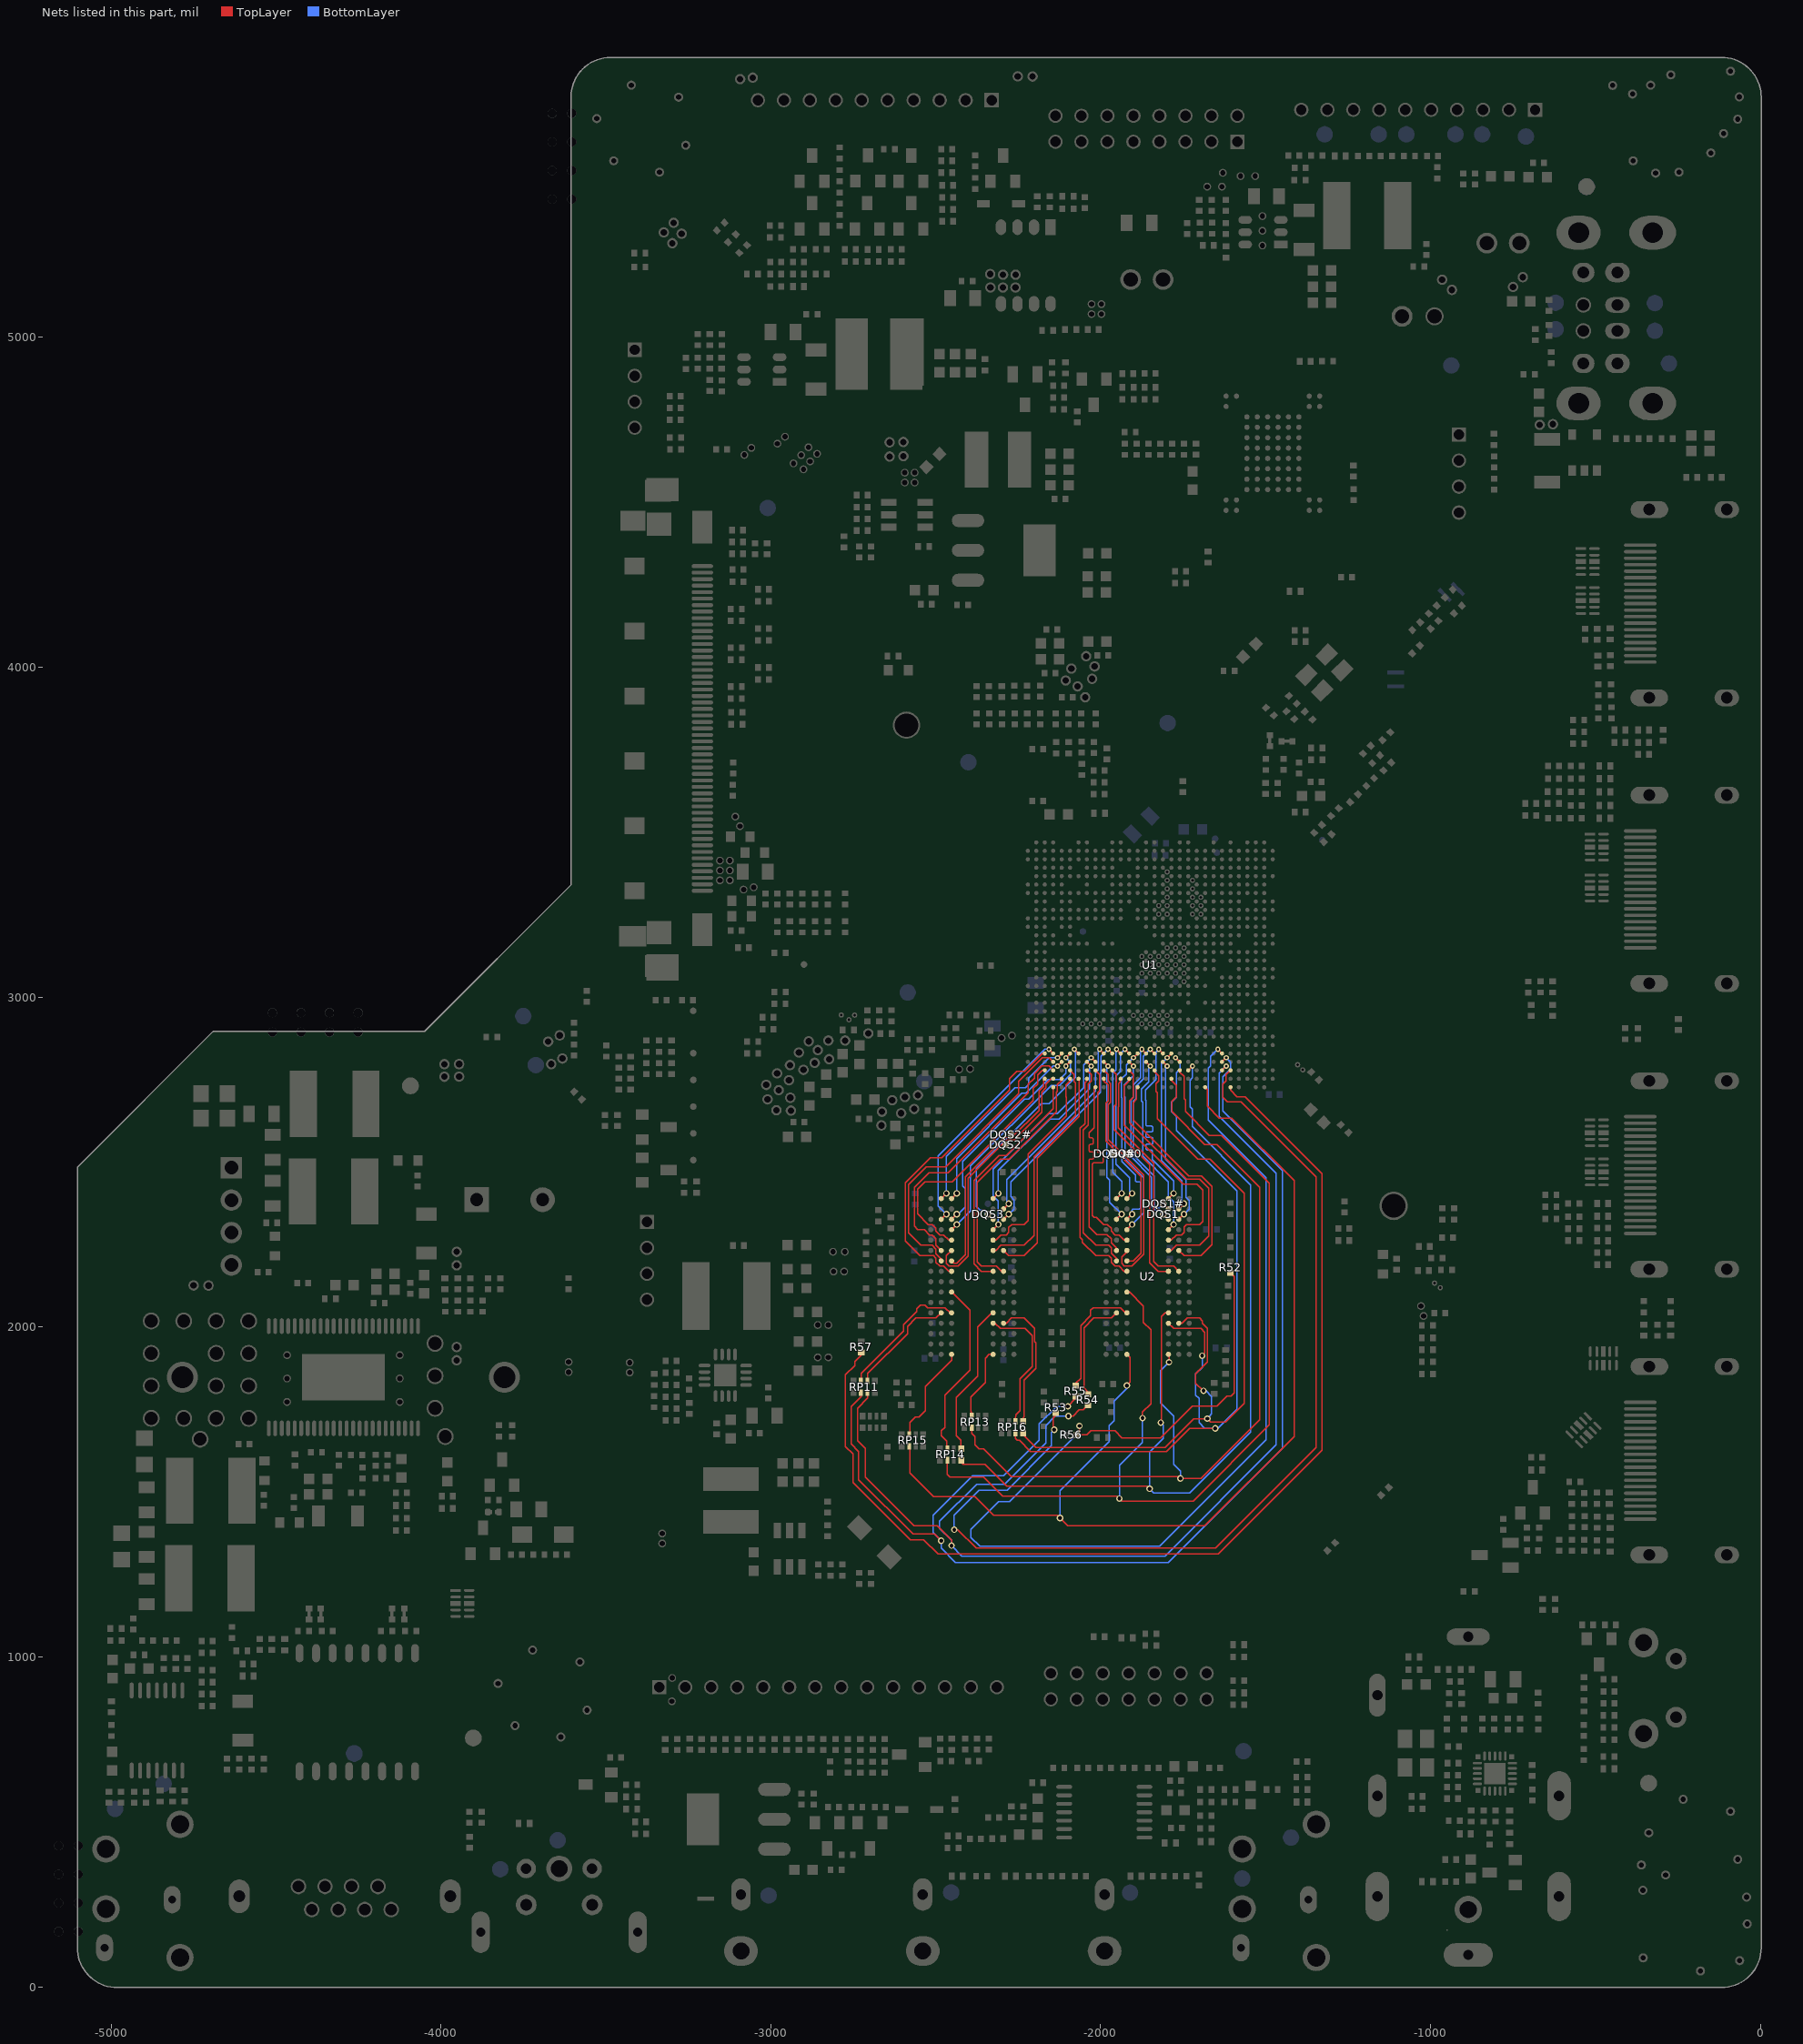
[diagram p0: the nets of this part, all layers, seen from the top]
# Altium PCB MISC86290.PcbDoc (part 12 of 31)
Units mil, origin at the board's own origin, x right, y up, seen from the top; angles counter-clockwise.
Board outline 5104.71 x 5851.49 mil, 2 copper layers (TopLayer, BottomLayer), stack 61.855 mil thick; 1026 components, 667 nets, 4280 pads, 2294 vias.

## Via types
v1: diameter 19.68, hole 11.81, TopLayer to BottomLayer, tented both sides, 1189 vias
v2: diameter 19.68/19.68 (per signal layer), hole 11.81, TopLayer to BottomLayer, tented both sides, 366 vias
v3: diameter 15.75, hole 7.87, TopLayer to BottomLayer, tented both sides, 348 vias
v4: diameter 23.62, hole 15.75, TopLayer to BottomLayer, tented both sides, 309 vias
v5: diameter 15.75/15.75 (per signal layer), hole 7.87, TopLayer to BottomLayer, tented both sides, 59 vias
v6: diameter 24/24 (per signal layer), hole 16, TopLayer to BottomLayer, tented both sides, 23 vias

## Nets (pads, with @x,y where several pads share a name; then routed paths per layer and width w, separated by ;. In a path a pad name is that pad's centre, name@x,y a point inside that pad or via, vN(x,y) a via of type N, cw(c..) or ccw(c..) an arc to the next point about the centre after c; other vN are vias at no path point) (continued)
D_DDR3_A12: RP16.4 U1.D12 U2.N7 | length 2408.7
  TopLayer w3.94: RP16.4@-2259.17,1678.74 -2259.17,1662.01 -2253.27,1656.1 -2246.38,1656.1 -2212.91,1622.64 -1800.51,1622.64 -1730.63,1692.52 v2(-1652.87,1692.52) ; U2.N7@-1794.61,2011.42 -1778.86,1995.67 -1696.18,1995.67 -1684.37,1983.86 -1684.37,1920.87 v2(-1692.24,1912.99) ; v5(-1772.95,2816.54) U1.D12@-1760.16,2803.74
  BottomLayer w3.94: v5(-1772.95,2816.54) -1759.17,2802.76 -1759.17,2783.07 -1770.98,2771.26 -1770.98,2696.46 -1785.75,2681.69 -1785.75,2653.15 -1770.98,2638.39 -1770.98,2596.06 -1586.93,2412.01 -1586.93,1750.59 -1645,1692.52 v2(-1652.87,1692.52) -1684.37,1692.52 -1702.09,1710.24 -1702.09,1783.07 -1711.93,1792.91 -1711.93,1857.87 -1692.24,1877.56 v2(-1692.24,1912.99)
D_DDR3_A12_H: RP16.3 U3.N7 | length 406.1
  TopLayer w3.94: U3.N7@-2326.1,2011.42 -2320.2,2011.42 -2304.45,1995.67 -2229.65,1995.67 -2207.99,1974.02 -2207.99,1879.53 -2244.41,1843.11 -2244.41,1746.65 -2257.2,1733.86 RP16.3@-2259.17,1722.05
D_DDR3_A13: RP15.6 U1.A9 U2.T3 | length 3206
  TopLayer w3.94: RP15.6@-2579.06,1638.39 -2579.06,1557.68 -2507.2,1485.83 -2381.22,1485.83 -2324.13,1428.74 -2131.22,1428.74 v2(-2123.35,1420.87) -2099.72,1397.24 -1684.37,1397.24 -1413.7,1667.91 -1413.7,2443.5 -1603.66,2633.46 -1641.06,2633.46 -1677.27,2669.68 -1677.27,2686.35 -1676.5,2687.13 -1676.5,2720.08 U1.A9@-1683.39,2726.97 ; v2(-1920.59,1822.44) -1920,1823.82 -1910.75,1833.07 -1910.75,1907.09 U2.T3@-1920.59,1916.93
  BottomLayer w3.94: v2(-2123.35,1420.87) -2123.35,1503.54 -1974.72,1652.17 -1974.72,1701.38 -1959.96,1716.14 -1959.96,1775.2 -1920.59,1814.57 v2(-1920.59,1822.44)
D_DDR3_A13_H: RP15.5 U3.T3 | length 294.2
  TopLayer w3.94: RP15.5@-2579.06,1681.69 -2579.06,1710.24 -2562.32,1726.97 -2551.5,1726.97 -2531.81,1746.65 -2531.81,1819.49 -2452.09,1899.21 U3.T3@-2452.09,1916.93
D_DDR3_A14: RP13.6 U1.B13 U2.T7 | length 2625.8
  TopLayer w3.94: RP13.6@-2391.06,1694.49 -2391.06,1677.76 -2381.22,1667.91 -2381.22,1643.31 -2368.43,1630.51 -2355.63,1630.51 -2270.98,1545.87 -1763.11,1545.87 v2(-1758.19,1540.94) -1696.18,1540.94 -1518.03,1719.09 -1518.03,2423.82 -1646.97,2552.76 -1684.37,2552.76 -1784.76,2653.15 -1784.76,2684.65 -1770.98,2698.43 -1770.98,2732.91 U1.B13@-1785.71,2747.64 ; U2.T7@-1794.61,1916.93 -1792.64,1916.93 v2(-1792.64,1893.31) ; U1.B13@-1785.75,2747.64 U1.B13@-1785.75,2752.56
  BottomLayer w3.94: v2(-1792.64,1893.31) -1818.23,1867.72 -1818.23,1769.29 -1778.86,1729.92 -1778.86,1583.27 -1758.19,1562.6 v2(-1758.19,1540.94)
D_DDR3_A14_H: RP13.5 U3.T7 | length 215.4
  TopLayer w3.94: RP13.5@-2391.06,1737.8 -2391.06,1740.07 -2394.02,1743.02 -2394.02,1787.99 -2349.72,1832.28 -2349.72,1905.12 -2337.91,1916.93 U3.T7@-2326.1,1916.93
D_DDR3_A15: RP14.2 U1.C11 U2.M7 | length 2781
  TopLayer w3.94: RP14.2@-2423.54,1596.06 -2423.54,1590.16 -2416.65,1583.27 -2350.71,1583.27 -2284.76,1517.32 -1859.57,1517.32 v2(-1851.69,1509.45) ; v2(-1818.23,1710.24) -1816.26,1707.36 -1816.26,2031.1 -1804.45,2042.91 U2.M7@-1794.61,2042.91 ; U1.C11@-1734.57,2778.15 v5(-1721.77,2790.94)
  BottomLayer w3.94: v2(-1818.23,1710.24) -1810.35,1702.36 -1810.35,1662.01 -1851.69,1620.67 v2(-1851.69,1509.45) -1838.9,1496.65 -1730.63,1496.65 -1545.59,1681.69 -1545.59,2430.71 -1722.76,2607.87 -1722.76,2660.04 -1729.65,2666.93 -1729.65,2747.64 -1721.77,2755.51 v5(-1721.77,2790.94)
D_DDR3_A15_H: RP14.1 U3.M7 | length 458.4
  TopLayer w3.94: RP14.1@-2423.54,1639.37 -2423.54,1656.1 -2438.31,1670.87 -2438.31,1786.02 -2373.35,1850.98 -2373.35,1999.61 -2330.04,2042.91 U3.M7@-2326.1,2042.91
D_DDR3_BA0: R54.2 RP11.4 U1.C7 | length 3734.8
  TopLayer w3.94: RP11.4@-2706.02,1800.79 -2706.02,1785.04 -2737.5,1753.56 -2737.5,1655.1 -2713.9,1631.5 -2713.9,1544.88 -2566.26,1397.24 -2495.39,1397.24 -2452.09,1353.94 v2(-2452.09,1337.2) ; v2(-2097.76,1729.92) -2083.98,1729.92 -2065.3,1748.6 -2053.18,1748.6 R54.2@-2038.7,1763.07 ; U1.C7@-1632.2,2778.15 v3(-1619.41,2790.94)
  BottomLayer w3.94: v2(-2097.76,1729.92) -2138.11,1729.92 -2166.65,1701.38 -2166.65,1648.23 -2291.65,1523.23 -2376.3,1523.23 -2488.5,1411.02 -2488.5,1389.37 -2452.09,1352.95 v2(-2452.09,1337.2) -2420.59,1305.71 -1805.43,1305.71 -1468.82,1642.32 -1468.82,2466.14 -1641.06,2638.39 -1641.06,2769.29 v3(-1619.41,2790.94)
D_DDR3_BA0_H: RP11.3 U3.M2 | length 326.7
  TopLayer w3.94: RP11.3@-2706.02,1844.09 -2706.02,1859.84 -2585.94,1979.92 -2585.94,2001.57 -2560.35,2027.17 -2499.33,2027.17 U3.M2@-2483.58,2042.91
D_DDR3_BA0_L: R54.1 U2.M2 | length 316.6
  TopLayer w3.94: R54.1@-2038.7,1803.07 -2050.51,1814.88 -2050.51,1997.64 -2020.98,2027.17 -1967.83,2027.17 U2.M2@-1952.09,2042.91
D_DDR3_BA1: RP16.2 U1.C15 U2.N8 | length 2335
  TopLayer w3.94: RP16.2@-2236.54,1678.74 -2236.52,1678.64 -2236.07,1674.34 -2196.18,1634.45 -1805.43,1634.45 -1717.83,1722.05 v2(-1676.5,1722.05) -1666.65,1712.2 -1621.38,1712.2 -1565.28,1768.31 -1565.28,2406.1 -1668.62,2509.45 -1706.02,2509.45 -1828.07,2631.5 -1828.07,2710.24 -1832.5,2714.67 -1832.5,2737.3 -1824.13,2745.67 -1824.13,2761.42 -1836.93,2774.21 U1.C15@-1836.93,2778.15 ; U2.N8@-1763.11,2011.42 -1753.27,2011.42 -1737.52,2027.17 -1700.12,2027.17 -1691.26,2018.31 -1691.26,2010.43 -1676.5,1995.67 -1676.5,1893.31 -1711.93,1857.87 -1711.93,1829.33 -1689.29,1806.69 v2(-1688.31,1806.69)
  BottomLayer w3.94: v2(-1688.31,1806.69) -1681.42,1806.69 -1663.7,1788.98 -1663.7,1736.81 v2(-1676.5,1722.05)
D_DDR3_BA1_H: RP16.1 U3.N8 | length 405.8
  TopLayer w3.94: U3.N8@-2294.61,2011.42 -2286.73,2011.42 -2270.98,2027.17 -2231.61,2027.17 -2200.12,1995.67 -2200.12,1956.3 -2196.18,1952.36 -2196.18,1874.61 -2232.6,1838.19 -2232.6,1726.97 -2234.57,1725 RP16.1@-2236.54,1722.05
D_DDR3_BA2: R55.2 RP11.6 U1.D7 | length 3823.5
  TopLayer w3.94: RP11.6@-2725.71,1800.79 -2725.71,1788.98 -2756.22,1758.46 -2756.22,1645.28 -2733.58,1622.64 -2733.58,1537.01 -2569.21,1372.64 -2504.25,1372.64 v2(-2483.58,1351.97) ; v2(-2099.72,1759.45) -2076.1,1783.07 R55.2@-2076.1,1788.66 ; U1.D7@-1632.2,2803.74 v5(-1619.41,2816.54)
  BottomLayer w3.94: v2(-2099.72,1759.45) -2133.19,1759.45 -2186.34,1706.3 -2186.34,1657.09 -2294.11,1549.31 -2387.62,1549.31 -2508.19,1428.74 -2508.19,1376.57 v2(-2483.58,1351.97) -2483.58,1329.33 -2440.28,1286.02 -1795.59,1286.02 -1449.13,1632.48 -1449.13,2475 -1629.25,2655.12 -1629.25,2758.46 -1605.63,2782.09 -1605.63,2802.76 v5(-1619.41,2816.54)
D_DDR3_BA2_H: RP11.5 U3.M3 | length 397
  TopLayer w3.94: RP11.5@-2725.72,1844.11 -2725.72,1859.83 -2597.76,1987.8 -2597.76,2007.48 -2558.39,2046.85 -2558.39,2054.72 -2546.57,2066.54 -2532.8,2066.54 -2524.92,2058.66 -2471.77,2058.66 U3.M3@-2456.02,2042.91
D_DDR3_BA2_L: R55.1 U2.M3 | length 360.9
  TopLayer w3.94: R55.1@-2076.1,1828.66 -2060.35,1844.41 -2060.35,2004.53 -2030.83,2034.06 -2030.83,2050.79 -2022.95,2058.66 -1940.28,2058.66 -1924.53,2042.91 U2.M3@-1920.59,2042.91
D_DDR3_CASZ: RP14.6 U1.C12 U2.K3 | length 3058.9
  TopLayer w3.94: RP14.6@-2465.87,1596.06 -2465.87,1553.74 -2457.01,1544.88 -2354.65,1544.88 -2297.56,1487.8 -1951.1,1487.8 v2(-1943.23,1479.92) -1935.35,1472.05 -1719.8,1472.05 -1488.5,1703.35 -1488.5,2435.63 -1633.19,2580.31 -1670.59,2580.31 -1743.43,2653.15 -1743.43,2688.58 -1747.36,2692.52 -1747.36,2759.45 -1760.16,2772.24 U1.C12@-1760.16,2778.15 ; U2.K3@-1920.59,2105.91 -1912.72,2105.91 -1870.39,2063.58 -1870.39,2014.37 -1847.76,1991.73 -1847.76,1767.32 -1873.35,1741.73 v2(-1873.35,1724.02)
  BottomLayer w3.94: v2(-1943.23,1479.92) -1943.23,1580.31 -1874.33,1649.21 -1874.33,1723.03 v2(-1873.35,1724.02)
D_DDR3_CASZ_H: RP14.5 U3.K3 | length 532.3
  TopLayer w3.94: RP14.5@-2465.87,1639.37 -2466.86,1639.37 -2466.86,1654.14 -2482.6,1669.88 -2482.6,1685.63 -2472.76,1695.47 -2472.76,1793.9 -2396.97,1869.69 -2396.97,2050.79 U3.K3@-2452.09,2105.91
D_DDR3_CKE: R52.2 R56.1 U1.E7 | length 3759
  TopLayer w3.94: v2(-2064.29,1700.39) -2064.29,1674.49 -2065.94,1672.83 -2042.64,1672.83 -2029.84,1685.63 -1957.01,1685.63 -1935.35,1663.98 -1818.23,1663.98 -1721.77,1760.43 -1647.95,1760.43 -1617.44,1790.94 -1604.65,1790.94 -1594.8,1800.79 -1594.8,2153.15 -1605.63,2163.98 -1605.94,2163.98 R52.2@-1606.61,2164.65 ; v5(-1645,2842.13) U1.E7@-1632.2,2829.33
  BottomLayer w3.94: v2(-2064.29,1700.39) -2064.29,1682.68 -2276.89,1470.08 -2309.37,1470.08 -2393.03,1386.42 -2393.03,1361.81 -2366.46,1335.24 -1821.18,1335.24 -1498.35,1658.07 -1498.35,2452.36 -1673.54,2627.56 -1673.54,2785.04 -1666.65,2791.93 -1666.65,2820.47 v5(-1645,2842.13)
D_DDR3_CSB1: R53.2 U1.C6 | length 3069.4
  TopLayer w3.94: v2(-2444.21,1385.43) -2433.39,1385.43 -2377.28,1329.33 -1651.89,1329.33 -1346.77,1634.45 -1346.77,2455.31 -1574.13,2682.68 -1615.47,2682.68 -1629.25,2696.46 -1629.25,2735.83 -1619.41,2745.67 -1619.41,2765.35 U1.C6@-1606.61,2778.15 ; v2(-2141.06,1688.58) -2144.69,1688.58 -2144.69,1724.02 R53.2@-2137.13,1731.57
  BottomLayer w3.94: v2(-2444.21,1385.43) -2444.21,1429.72 -2368.43,1505.51 -2283.78,1505.51 -2148.94,1640.35 -2148.94,1680.71 v2(-2141.06,1688.58)
D_DDR3_CSB2: R57.1 U1.A6 | length 3289.4
  TopLayer w3.94: R57.1@-2724.72,1916.2 -2745.39,1895.53 -2745.39,1883.46 -2773.94,1854.92 -2773.94,1637.4 -2751.3,1614.76 -2751.3,1529.13 -2577.09,1354.92 -2536.73,1354.92 -2493.43,1311.61 -1644.02,1311.61 -1329.06,1626.57 -1329.06,2465.16 -1562.32,2698.43 -1586.93,2698.43 -1606.61,2718.11 U1.A6@-1606.61,2726.97
D_DDR3_DM0: U1.B18 U2.E7 | length 700.1
  TopLayer w3.94: U1.B18@-1913.7,2752.56 -1913.7,2746.65 -1929.45,2730.91 -1929.45,2611.81 -1750.32,2432.68 -1707.99,2432.68 -1690.28,2414.96 -1690.28,2320.47 -1700.12,2310.63 -1740.28,2310.63 -1747.36,2303.55 -1747.36,2287.01 -1755.24,2279.13 -1770.98,2279.13 -1786.73,2263.39 U2.E7@-1794.61,2263.39
D_DDR3_DM1: U1.D18 U2.D3 | length 571.2
  TopLayer w3.94: U2.D3@-1920.59,2294.88 v2(-1904.84,2310.63) ; U1.D18@-1913.7,2803.74 v5(-1900.91,2790.94)
  BottomLayer w3.94: v2(-1904.84,2310.63) -1869.41,2346.06 -1869.41,2452.36 -1926.5,2509.45 -1926.5,2697.44 -1928.46,2699.41 -1928.46,2733.86 -1900.91,2761.42 v5(-1900.91,2790.94)
D_DDR3_DM2: U1.B25 U3.E7 | length 622.8
  TopLayer w3.94: U3.E7@-2326.1,2263.39 -2318.23,2263.39 -2302.48,2279.13 -2286.73,2279.13 -2278.86,2287.01 -2278.86,2301.5 -2269.73,2310.63 -2231.61,2310.63 -2219.8,2322.44 -2219.8,2524.21 -2104.65,2639.37 -2104.65,2696.46 -2105.63,2697.44 -2105.63,2733.86 -2092.83,2746.65 U1.B25@-2092.83,2752.56
D_DDR3_DM3: U1.E25 U3.D3 | length 709.7
  TopLayer w3.94: U3.D3@-2452.09,2294.88 v2(-2436.34,2310.63) ; v5(-2105.63,2816.54) U1.E25@-2092.83,2829.33
  BottomLayer w3.94: v2(-2436.34,2310.63) -2395,2351.97 -2395,2487.8 -2149.92,2732.87 -2124.33,2732.87 -2091.85,2765.35 -2091.85,2802.76 v5(-2105.63,2816.54)
D_DDR3_DQ0: U1.C22 U2.E3 | length 630.1
  TopLayer w3.94: U1.C22@-2016.06,2778.15 -2003.27,2765.35 -2003.27,2716.14 -2009.17,2710.24 -2009.17,2532.9 ccw(c-2005.24,2532.9) -2005.24,2528.96 -1996.38,2528.96 cw(c-1996.38,2525.02) -1992.44,2525.02 -1992.44,2501.57 cw(c-1996.38,2501.57) -1996.38,2497.64 -2020.99,2497.64 ccw(c-2020.98,2493.7) -2024.92,2493.7 -2024.92,2338.19 -2019.51,2332.78 -2013.6,2332.78 -1991.46,2310.63 -1979.65,2310.63 -1967.83,2298.82 -1967.83,2290.94 -1956.02,2279.13 -1944.21,2279.13 -1928.46,2263.39 U2.E3@-1920.59,2263.39
D_DDR3_DQ1: U1.C18 U2.F7 | length 775.4
  TopLayer w3.94: U1.C18@-1913.7,2778.15 -1900.91,2765.35 -1900.91,2696.46 -1911.73,2685.63 -1911.73,2619.68 -1740.47,2448.43 -1700.12,2448.43 -1672.56,2420.87 -1672.56,2275.2 -1700.12,2247.64 -1770.98,2247.64 -1786.73,2231.89 U2.F7@-1794.61,2231.89
D_DDR3_DQ2: U1.A22 U2.F2 | length 592.6
  TopLayer w3.94: U1.A22@-2016.06,2726.97 -2019.51,2723.52 -2019.51,2604.43 -2034.76,2589.17 -2034.76,2577.36 ccw(c-2030.83,2577.36) -2030.83,2573.43 -2026.89,2573.43 cw(c-2026.89,2569.49) -2022.95,2569.49 -2022.95,2557.68 cw(c-2026.89,2557.68) -2026.89,2553.74 -2030.84,2553.74 ccw(c-2030.83,2549.8) -2034.76,2549.8 -2034.76,2535.04 ccw(c-2030.83,2535.04) -2030.83,2531.1 -2024.92,2531.1 cw(c-2024.92,2527.17) -2020.98,2527.17 -2020.98,2513.39 cw(c-2024.92,2513.39) -2024.92,2509.45 -2030.84,2509.45 ccw(c-2030.83,2505.51) -2034.76,2505.51 -2034.76,2303.74 -2011.19,2280.17 -1980.68,2280.17 -1967.83,2267.32 -1967.83,2255.51 -1952.09,2239.76 U2.F2@-1952.09,2231.89
D_DDR3_DQ3: U1.A17 U2.F8 | length 725.4
  TopLayer w3.94: U1.A17@-1888.11,2726.97 -1891.06,2724.02 -1891.06,2690.55 -1901.89,2679.72 -1901.89,2627.56 -1732.6,2458.27 -1694.21,2458.27 -1662.72,2426.77 -1662.72,2249.61 -1696.18,2216.14 -1747.36,2216.14 U2.F8@-1763.11,2231.89
D_DDR3_DQ4: U1.B23 U2.H3 | length 685.5
  TopLayer w3.94: U1.B23@-2041.65,2752.56 -2041.65,2746.65 -2047.56,2740.75 -2047.56,2616.73 -2062.32,2601.97 -2062.32,2271.26 -2055.43,2264.37 -2055.43,2256.5 -2015.08,2216.14 -1975.71,2216.14 -1967.83,2208.27 -1967.83,2196.46 -1956.02,2184.65 -1944.21,2184.65 -1928.46,2168.9 U2.H3@-1920.59,2168.9
D_DDR3_DQ5: U1.B19 U2.H8 | length 690.8
  TopLayer w3.94: U1.B19@-1939.29,2752.56 -1939.29,2744.68 -1946.16,2737.81 -1946.16,2667.93 -1947.17,2666.93 -1947.17,2603.94 -1839.88,2496.65 -1839.88,2198.43 -1826.1,2184.65 -1778.86,2184.65 U2.H8@-1763.11,2168.9
D_DDR3_DQ6: U1.C23 U2.G2 | length 657.5
  TopLayer w3.94: U1.C23@-2041.65,2778.15 -2028.86,2765.35 -2028.86,2745.67 -2037.72,2736.81 -2037.72,2611.81 -2052.48,2597.05 -2052.48,2285.04 -2015.08,2247.64 -1975.71,2247.64 -1967.83,2239.76 -1967.83,2224.02 -1952.09,2208.27 U2.G2@-1952.09,2200.39
D_DDR3_DQ7: U1.C20 U2.H7 | length 703.9
  TopLayer w3.94: U1.C20@-1964.88,2778.15 -1952.09,2765.35 -1952.09,2743.7 -1954,2741.79 -1954,2673.87 -1958.98,2668.9 -1958.98,2599.02 -1851.69,2491.73 -1851.69,2194.49 -1826.1,2168.9 U2.H7@-1794.61,2168.9
D_DDR3_DQ8: U1.D16 U2.D7 | length 572.1
  TopLayer w3.94: U1.D16@-1862.52,2803.74 v5(-1849.72,2790.94) ; U2.D7@-1794.61,2294.88 v2(-1778.86,2310.63)
  BottomLayer w3.94: v5(-1849.72,2790.94) -1854.65,2786.02 -1854.65,2742.72 -1876.3,2721.06 -1876.3,2685.63 -1872.36,2681.69 -1872.36,2518.31 -1794.61,2440.55 -1794.61,2395.28 -1778.86,2379.53 v2(-1778.86,2310.63)
D_DDR3_DQ9: U1.E17 U2.C3 | length 582
  TopLayer w3.94: U2.C3@-1920.59,2326.38 v2(-1904.84,2342.13) ; v5(-1900.91,2816.54) U1.E17@-1888.11,2829.33
  BottomLayer w3.94: v2(-1904.84,2342.13) -1904.84,2353.94 cw(c-1900.91,2353.94) -1900.91,2357.87 -1883.19,2357.87 ccw(c-1883.19,2361.81) -1879.25,2361.81 -1879.25,2436.61 ccw(c-1883.19,2436.61) -1883.19,2440.55 -1891.06,2440.55 cw(c-1891.06,2444.49) -1895,2444.49 -1895,2460.24 -1936.34,2501.57 -1936.34,2694.49 -1937.32,2695.47 -1937.32,2752.56 -1922.56,2767.32 -1922.56,2794.88 v5(-1900.91,2816.54)
D_DDR3_DQ10: U1.D14 U2.C8 | length 527.5
  TopLayer w3.94: U1.D14@-1811.34,2803.74 v5(-1798.54,2790.94) ; U2.C8@-1763.11,2326.38 v2(-1747.36,2342.13)
  BottomLayer w3.94: v5(-1798.54,2790.94) -1803.46,2786.02 -1803.46,2509.45 -1741.46,2447.44 -1741.46,2393.31 -1731.61,2383.46 -1731.61,2357.87 v2(-1747.36,2342.13)
D_DDR3_DQ11: U1.D21 U2.C2 | length 509.6
  TopLayer w3.94: U1.D21@-1990.47,2803.74 v5(-1977.68,2790.94) ; U2.C2@-1952.09,2326.38 v2(-1936.34,2342.13)
  BottomLayer w3.94: v5(-1977.68,2790.94) -1981.61,2787.01 -1981.61,2454.33 -1972.76,2445.47 -1972.76,2378.54 v2(-1936.34,2342.13)
D_DDR3_DQ12: U1.E14 U2.A7 | length 606.6
  TopLayer w3.94: v5(-1824.13,2842.13) U1.E14@-1811.34,2829.33 ; U2.A7@-1794.61,2389.37 v2(-1778.86,2405.12)
  BottomLayer w3.94: v5(-1824.13,2842.13) -1832.99,2833.27 -1832.99,2749.61 -1864.49,2718.11 -1864.49,2688.58 -1862.52,2686.61 -1862.52,2612.8 ccw(c-1858.58,2612.8) -1858.58,2608.86 -1845.79,2608.86 cw(c-1845.79,2604.92) -1841.85,2604.92 -1841.85,2596.06 cw(c-1845.79,2596.06) -1845.79,2592.13 -1858.58,2592.13 ccw(c-1858.58,2588.19) -1862.52,2588.19 -1862.52,2578.35 ccw(c-1858.58,2578.35) -1858.58,2574.41 -1845.79,2574.41 cw(c-1845.79,2570.47) -1841.85,2570.47 -1841.85,2558.66 cw(c-1845.79,2558.66) -1845.79,2554.72 -1858.58,2554.72 ccw(c-1858.58,2550.79) -1862.52,2550.79 -1862.52,2540.94 ccw(c-1858.58,2540.94) -1858.58,2537.01 -1847.26,2537.01 cw(c-1847.26,2533.07) -1843.33,2533.07 -1843.33,2506.99 -1778.86,2442.52 v2(-1778.86,2405.12)
D_DDR3_DQ13: U1.E19 U2.A2 | length 493.7
  TopLayer w3.94: U2.A2@-1952.09,2389.37 v2(-1936.34,2405.12) ; v5(-1952.09,2842.13) U1.E19@-1939.29,2829.33
  BottomLayer w3.94: v5(-1952.09,2842.13) -1954.06,2840.16 -1954.06,2779.13 -1963.9,2769.29 -1963.9,2469.09 -1936.34,2441.54 v2(-1936.34,2405.12)
D_DDR3_DQ14: U1.E13 U2.B8 | length 518.3
  TopLayer w3.94: v5(-1798.54,2816.54) U1.E13@-1785.75,2829.33 ; U2.B8@-1763.11,2357.87 v2(-1747.36,2373.62)
  BottomLayer w3.94: v5(-1798.54,2816.54) -1815.28,2799.8 -1815.28,2504.53 -1753.27,2442.52 -1753.27,2379.53 v2(-1747.36,2373.62)
D_DDR3_DQ15: U1.E18 U2.A3 | length 509.2
  TopLayer w3.94: v5(-1926.5,2842.13) U1.E18@-1913.7,2829.33 ; U2.A3@-1920.59,2389.37 v2(-1904.84,2405.12)
  BottomLayer w3.94: v5(-1926.5,2842.13) -1940.28,2828.35 -1940.28,2775.2 -1954.06,2761.42 -1954.06,2493.7 -1912.72,2452.36 -1912.72,2412.99 v2(-1904.84,2405.12)
D_DDR3_DQ16: U1.C28 U3.E3 | length 788.3
  TopLayer w3.94: U3.E3@-2452.09,2263.39 -2459.96,2263.39 -2475.71,2279.13 -2487.52,2279.13 -2499.33,2290.94 -2499.33,2298.82 -2511.14,2310.63 -2522.95,2310.63 -2555.43,2343.11 -2555.43,2417.91 -2532.8,2440.55 -2450.12,2440.55 -2204.06,2686.61 -2204.06,2724.02 -2191.26,2736.81 -2191.26,2763.39 -2176.5,2778.15 U1.C28@-2169.61,2778.15
D_DDR3_DQ17: U1.C25 U3.F7 | length 702.1
  TopLayer w3.94: U3.F7@-2326.1,2231.89 -2318.23,2231.89 -2302.48,2247.64 -2231.61,2247.64 -2202.09,2277.17 -2202.09,2516.34 -2077.09,2641.34 -2077.09,2740.75 -2080.04,2743.7 -2080.04,2765.35 U1.C25@-2092.83,2778.15
D_DDR3_DQ18: U1.C27 U3.F2 | length 843.6
  TopLayer w3.94: U3.F2@-2483.58,2231.89 -2499.33,2247.64 -2499.33,2267.32 -2511.14,2279.13 -2519.02,2279.13 -2534.76,2294.88 -2554.45,2294.88 -2565.28,2305.71 -2565.28,2423.82 -2520.98,2468.11 -2461.93,2468.11 -2219.8,2710.24 -2219.8,2735.83 -2201.1,2754.53 -2201.1,2768.31 -2178.46,2790.94 -2156.81,2790.94 U1.C27@-2144.02,2778.15
D_DDR3_DQ19: U1.B24 U3.F8 | length 675.6
  TopLayer w3.94: U3.F8@-2294.61,2231.89 -2278.86,2216.14 -2231.61,2216.14 -2192.24,2255.51 -2192.24,2511.42 -2065.28,2638.39 -2065.28,2750.59 U1.B24@-2067.24,2752.56
D_DDR3_DQ20: U1.E28 U3.H3 | length 967.8
  TopLayer w3.94: U3.H3@-2452.09,2168.9 -2459.96,2168.9 -2475.71,2184.65 -2487.52,2184.65 -2499.33,2196.46 -2499.33,2208.27 -2507.2,2216.14 -2548.54,2216.14 -2592.83,2260.43 -2592.83,2436.61 -2516.06,2513.39 -2481.61,2513.39 -2275.91,2719.09 -2275.91,2753.54 -2253.76,2775.69 -2231.12,2775.69 -2177.48,2829.33 U1.E28@-2169.61,2829.33
D_DDR3_DQ21: U1.B26 U3.H8 | length 768.2
  TopLayer w3.94: U3.H8@-2294.61,2168.9 -2300.51,2168.9 -2316.26,2184.65 -2361.54,2184.65 -2374.33,2197.44 -2374.33,2438.58 -2304.45,2508.46 -2277.87,2508.46 -2134.17,2652.17 -2134.17,2711.22 -2131.22,2714.17 -2131.22,2734.84 -2118.43,2747.64 U1.B26@-2118.43,2752.56
D_DDR3_DQ22: U1.D27 U3.G2 | length 917.7
  TopLayer w3.94: U3.G2@-2483.58,2200.39 -2483.58,2205.82 -2499.33,2221.56 -2499.33,2235.83 -2511.14,2247.64 -2544.61,2247.64 -2582.99,2286.02 -2582.99,2431.69 -2528.86,2485.83 -2469.8,2485.83 -2248.35,2707.28 -2248.35,2744.68 -2176.5,2816.54 -2156.81,2816.54 U1.D27@-2144.02,2803.74
D_DDR3_DQ23: U1.A27 U3.H7 | length 715
  TopLayer w3.94: U3.H7@-2326.1,2168.9 -2361.54,2168.9 -2384.17,2191.54 -2384.17,2443.5 -2308.39,2519.29 -2286.73,2519.29 -2144.02,2662.01 U1.A27@-2144.02,2726.97
D_DDR3_DQ24: U1.D22 U3.D7 | length 691.5
  TopLayer w3.94: U3.D7@-2326.1,2294.88 v2(-2310.35,2310.63) ; v5(-2028.86,2816.54) U1.D22@-2016.06,2803.74
  BottomLayer w3.94: v2(-2310.35,2310.63) -2310.35,2381.5 -2326.1,2397.24 -2326.1,2477.95 -2157.8,2646.26 -2131.22,2646.26 -2051.5,2725.98 -2051.5,2793.9 v5(-2028.86,2816.54)
D_DDR3_DQ25: U1.D25 U3.C3 | length 662.1
  TopLayer w3.94: U3.C3@-2452.09,2326.38 v2(-2436.34,2342.13) ; v5(-2105.63,2790.94) U1.D25@-2092.83,2803.74
  BottomLayer w3.94: v2(-2436.34,2342.13) -2432.4,2342.13 -2410.75,2363.78 -2410.75,2419.88 -2418.62,2427.76 -2418.62,2502.56 -2230.63,2690.55 -2218.82,2690.55 -2158.78,2750.59 -2124.33,2750.59 -2105.63,2769.29 v5(-2105.63,2790.94)
D_DDR3_DQ26: U1.E20 U3.C8 | length 673.3
  TopLayer w3.94: U3.C8@-2294.61,2326.38 v2(-2278.86,2342.13) ; v5(-1977.68,2842.13) U1.E20@-1964.88,2829.33
  BottomLayer w3.94: v2(-2278.86,2342.13) -2263.11,2357.87 -2263.11,2385.43 -2272.95,2395.28 -2272.95,2439.57 -2000.32,2712.2 -2000.32,2770.28 -1999.33,2771.26 -1999.33,2820.47 v5(-1977.68,2842.13)
D_DDR3_DQ27: U1.E27 U3.C2 | length 696.5
  TopLayer w3.94: U3.C2@-2483.58,2326.38 v2(-2467.83,2342.13) ; v5(-2156.81,2842.13) U1.E27@-2144.02,2829.33
  BottomLayer w3.94: v2(-2467.83,2342.13) -2492.44,2366.73 -2492.44,2518.31 -2168.62,2842.13 v5(-2156.81,2842.13)
D_DDR3_DQ28: U1.D23 U3.A7 | length 558.9
  TopLayer w3.94: U3.A7@-2326.1,2389.37 v2(-2310.35,2405.12) ; U1.D23@-2041.65,2803.74 v5(-2028.86,2790.94)
  BottomLayer w3.94: v2(-2310.35,2405.12) -2310.35,2474.02 -2153.86,2630.51 -2126.3,2630.51 -2034.27,2722.54 -2034.27,2785.53 v5(-2028.86,2790.94)
D_DDR3_DQ29: U1.E26 U3.A2 | length 624.7
  TopLayer w3.94: U3.A2@-2483.58,2389.37 v2(-2467.83,2405.12) ; v5(-2131.22,2816.54) U1.E26@-2118.43,2829.33
  BottomLayer w3.94: v2(-2467.83,2405.12) -2467.83,2517.32 -2260.16,2725 -2228.66,2725 -2218.82,2734.84 -2218.82,2754.53 -2156.81,2816.54 v5(-2131.22,2816.54)
D_DDR3_DQ30: U1.E21 U3.B8 | length 627.9
  TopLayer w3.94: U3.B8@-2294.61,2357.87 v2(-2278.86,2373.62) ; v5(-2003.27,2842.13) U1.E21@-1990.47,2829.33
  BottomLayer w3.94: v2(-2278.86,2373.62) -2284.76,2379.53 -2284.76,2446.46 -2016.06,2715.16 -2016.06,2769.78 -2007.2,2778.64 -2007.2,2838.19 v5(-2003.27,2842.13)
D_DDR3_DQ31: U1.D26 U3.A3 | length 567
  TopLayer w3.94: U3.A3@-2452.09,2389.37 v2(-2436.34,2405.12) ; v5(-2131.22,2790.94) U1.D26@-2118.43,2803.74
  BottomLayer w3.94: v2(-2436.34,2405.12) -2436.34,2510.43 -2238.5,2708.27 -2226.69,2708.27 -2144.02,2790.94 v5(-2131.22,2790.94)
D_DDR3_DQS0: DQS0.1 U1.C21 U2.F3 | length 744.5
  TopLayer w3.94: U1.C21@-1990.47,2778.15 -1977.68,2765.35 -1977.68,2745.67 -1969.97,2737.96 -1969.97,2681.52 -1976.69,2674.8 -1976.69,2567.52 -1928.59,2519.41 -1869.41,2460.24 -1869.41,2220.08 -1904.84,2184.65 -1928.46,2184.65 -1936.34,2192.52 -1936.34,2212.2 -1920.59,2227.95 U2.F3@-1920.59,2231.89
D_DDR3_DQS0B: DQS0#.1 U1.B21 U2.G3 | length 634.1
  TopLayer w3.94: -1990.47,2745.67 U1.B21@-1990.47,2752.56 ; -1990.42,2745.67 -1977.81,2733.05 -1977.81,2685.5 -1984.57,2678.74 -1984.57,2563.58 -1951.99,2531.01 -1877.28,2456.3 -1877.28,2224.02 -1900.91,2200.39 U2.G3@-1920.59,2200.39
D_DDR3_DQS1: DQS1.1 U1.E16 U2.C7 | length 601.9
  TopLayer w3.94: v5(-1875.32,2842.13) U1.E16@-1862.52,2829.33 ; v2(-1810.35,2342.13) U2.C7@-1794.61,2326.38
  BottomLayer w3.94: v5(-1875.32,2842.13) -1879.25,2838.19 -1879.25,2755.51 -1900.91,2733.86 -1900.91,2696.46 -1908.78,2688.58 -1908.78,2517.32 -1845.79,2454.33 -1845.79,2365.75 -1833.98,2353.94 -1822.17,2353.94 v2(-1810.35,2342.13)
D_DDR3_DQS1B: DQS1#.1 U1.E15 U2.B7 | length 595.8
  TopLayer w3.94: v5(-1849.72,2842.13) U1.E15@-1836.93,2829.33 ; v2(-1810.35,2373.62) U2.B7@-1794.61,2357.87
  BottomLayer w3.94: v5(-1849.72,2842.13) -1871.38,2820.47 -1871.38,2751.57 -1893.03,2729.92 -1893.03,2692.52 -1900.91,2684.65 -1900.91,2521.26 -1837.91,2458.27 -1837.91,2369.69 -1830.04,2361.81 -1822.17,2361.81 v2(-1810.35,2373.62)
D_DDR3_DQS2: DQS2.1 U1.B27 U3.F3 | length 789.3
  TopLayer w3.94: U3.F3@-2452.09,2231.89 -2467.83,2216.14 -2467.83,2192.52 -2459.96,2184.65 -2432.4,2184.65 -2401.89,2215.16 -2401.89,2451.38 -2286.73,2566.54 -2263.11,2566.54 -2178.46,2651.18 -2178.46,2712.2 -2165.67,2725 -2165.67,2736.81 -2149.92,2752.56 U1.B27@-2144.02,2752.56
D_DDR3_DQS2B: DQS2#.1 U1.B28 U3.G3 | length 702.2
  TopLayer w3.94: U3.G3@-2452.09,2200.39 -2444.21,2192.52 -2436.34,2192.52 -2409.76,2219.09 -2409.76,2455.31 -2290.67,2574.41 -2269.02,2574.41 -2186.34,2657.09 -2186.34,2716.14 -2173.54,2728.94 -2173.54,2748.62 U1.B28@-2169.61,2752.56
D_DDR3_DQS3: DQS3.1 U1.E24 U3.C7 | length 702.2
  TopLayer w3.94: v2(-2341.85,2342.13) U3.C7@-2326.1,2326.38 ; v5(-2080.04,2842.13) U1.E24@-2067.24,2829.33
  BottomLayer w3.94: v2(-2341.85,2342.13) -2353.66,2353.94 -2365.47,2353.94 -2377.28,2365.75 -2377.28,2479.92 -2179.45,2677.76 -2155.83,2677.76 -2076.1,2757.48 -2076.1,2838.19 v5(-2080.04,2842.13)